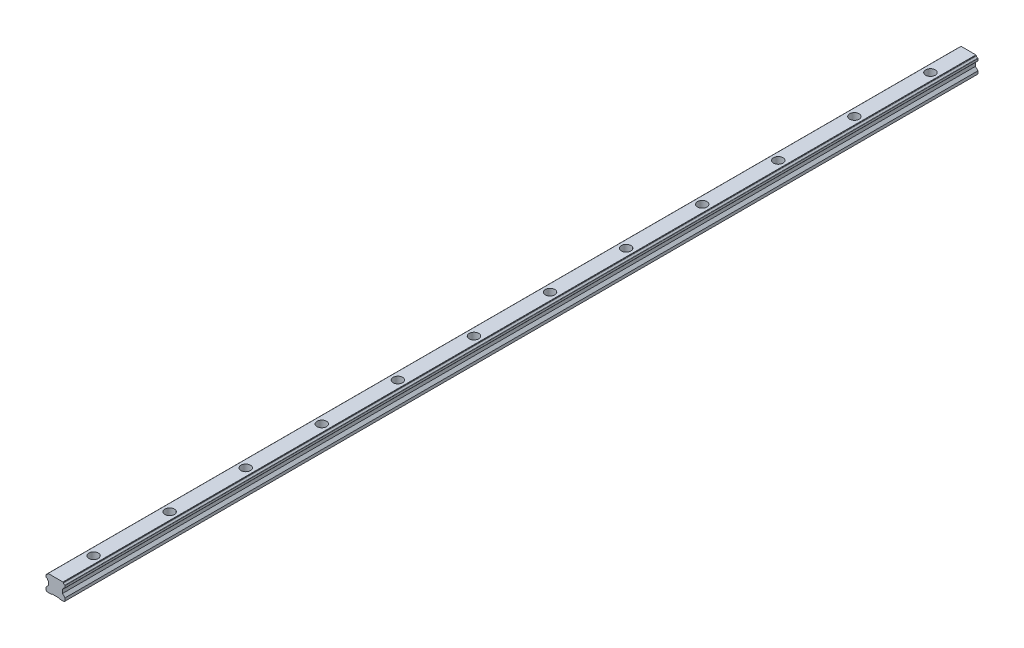
from build123d import *

# Parameters (mm, degrees)
BOSS_EXTRUDE1_DEPTH = 720
CUT_EXTRUDE1_DEPTH  = 721.116346502
CUT_EXTRUDE2_DEPTH  = 721.116346502
CUT_EXTRUDE3_DEPTH  = 721.116346502
CUT_EXTRUDE4_DEPTH  = 200
HOLE1_D             = 4.5
HOLE1_CBORE_D       = 7.5
HOLE1_CBORE_DEPTH   = 6
CHAMFER1_SIZE       = 0.7
CHAMFER2_SIZE       = 0.7
FILLET1_R           = 0.3
FILLET2_R           = 0.3
FILLET3_R           = 0.3
FILLET4_R           = 0.3
FILLET5_R           = 0.3
FILLET6_R           = 0.3
FILLET7_R           = 0.3
FILLET8_R           = 0.3
LPATTERN1_COUNT     = 12
LPATTERN1_PITCH     = 60


with BuildPart() as part:
    # Sketch1 → Boss-Extrude1 (new body)
    with BuildSketch(Plane.XY):
        with BuildLine():
            Line((7.5, -10.55), (7.5, 1.029661645))
            ThreePointArc((7.5, 1.029661645), (6.653187418, 1.325902711), (6.199900247, 2.100099753))
            Line((6.199900247, 2.100099753), (5.85, 2.45))
            Line((5.85, 2.45), (-5.85, 2.45))
            Line((-5.85, 2.45), (-6.199900248, 2.100099753))
            ThreePointArc((-6.199900248, 2.100099753), (-6.653187418, 1.325902711), (-7.5, 1.029661645))
            Line((-7.5, 1.029661645), (-7.5, -10.55))
            Line((-7.5, -10.55), (7.5, -10.55))
        make_face()
    extrude(amount=-BOSS_EXTRUDE1_DEPTH)

    # Sketch2 → Cut-Extrude1 (cut, through all)
    with BuildSketch(Plane(origin=(0, 0, -720), x_dir=(-1, 0, 0), z_dir=(0, 0, -1))):
        with BuildLine():
            Line((-7.5, -1.029661645), (-7.5, -7.6))
            Line((-7.5, -7.6), (-5.5, -5.6))
            Line((-5.5, -5.6), (-5.5, -2.8))
            Line((-5.5, -2.8), (-6.199900248, -2.100099752))
            ThreePointArc((-6.199900248, -2.100099752), (-6.653187419, -1.325902711), (-7.5, -1.029661645))
        make_face()
    extrude(amount=-CUT_EXTRUDE1_DEPTH, mode=Mode.SUBTRACT)

    # Sketch3 → Cut-Extrude2 (cut, through all)
    with BuildSketch(Plane(origin=(0, 0, -720), x_dir=(-1, 0, 0), z_dir=(0, 0, -1))):
        with BuildLine():
            Line((6.199900248, -2.100099752), (5.5, -2.8))
            Line((5.5, -2.8), (5.5, -5.6))
            Line((5.5, -5.6), (7.5, -7.6))
            Line((7.5, -7.6), (7.5, -1.029661645))
            ThreePointArc((7.5, -1.029661645), (6.653187419, -1.325902711), (6.199900248, -2.100099752))
        make_face()
    extrude(amount=-CUT_EXTRUDE2_DEPTH, mode=Mode.SUBTRACT)

    # Sketch4 → Cut-Extrude3 (cut, through all)
    with BuildSketch(Plane(origin=(0, 0, -720), x_dir=(-1, 0, 0), z_dir=(0, 0, -1))):
        Polygon((-3.35, -10.55), (3.35, -10.55), (2.85, -10.05), (-2.85, -10.05), align=None)
    extrude(amount=-CUT_EXTRUDE3_DEPTH, mode=Mode.SUBTRACT)

    # Sketch5 → Cut-Extrude4 (cut)
    with BuildSketch(Plane(origin=(0, 0, -720), x_dir=(-1, 0, 0), z_dir=(0, 0, -1))):
        with BuildLine():
            Line((-5.75, -10.55), (-4.95, -10.55))
            ThreePointArc((-4.95, -10.55), (-5.35, -10.35), (-5.75, -10.55))
        make_face()
    extrude(amount=-CUT_EXTRUDE4_DEPTH, mode=Mode.SUBTRACT)

    # Hole1 (through all)
    with Locations(Plane(origin=(0, 2.45, 0), x_dir=(-1, 0, 0), z_dir=(0, 1, 0))):
        with Locations((0, -30)):
            hole1 = CounterBoreHole(HOLE1_D / 2, HOLE1_CBORE_D / 2, HOLE1_CBORE_DEPTH)

    # Chamfer1
    chamfer1_edges = [part.edges().sort_by_distance(p)[0] for p in [
        (-7.5, -10.55, -360),
    ]]
    chamfer(chamfer1_edges, length=CHAMFER1_SIZE)

    # Chamfer2
    chamfer2_edges = [part.edges().sort_by_distance(p)[0] for p in [
        (7.5, -10.55, -360),
    ]]
    chamfer(chamfer2_edges, length=CHAMFER2_SIZE)

    # Fillet1
    fillet1_edges = [part.edges().sort_by_distance(p)[0] for p in [
        (7.5, 1.029661645, -360),
    ]]
    fillet(fillet1_edges, radius=FILLET1_R)

    # Fillet2
    fillet2_edges = [part.edges().sort_by_distance(p)[0] for p in [
        (-7.5, 1.029661645, -360),
    ]]
    fillet(fillet2_edges, radius=FILLET2_R)

    # Fillet3
    fillet3_edges = [part.edges().sort_by_distance(p)[0] for p in [
        (7.5, -1.029661645, -360),
    ]]
    fillet(fillet3_edges, radius=FILLET3_R)

    # Fillet4
    fillet4_edges = [part.edges().sort_by_distance(p)[0] for p in [
        (6.199900247, 2.100099753, -360),
    ]]
    fillet(fillet4_edges, radius=FILLET4_R)

    # Fillet5
    fillet5_edges = [part.edges().sort_by_distance(p)[0] for p in [
        (-7.5, -1.029661645, -360),
    ]]
    fillet(fillet5_edges, radius=FILLET5_R)

    # Fillet6
    fillet6_edges = [part.edges().sort_by_distance(p)[0] for p in [
        (-6.199900248, -2.100099752, -360),
    ]]
    fillet(fillet6_edges, radius=FILLET6_R)

    # Fillet7
    fillet7_edges = [part.edges().sort_by_distance(p)[0] for p in [
        (6.199900248, -2.100099752, -360),
    ]]
    fillet(fillet7_edges, radius=FILLET7_R)

    # Fillet8
    fillet8_edges = [part.edges().sort_by_distance(p)[0] for p in [
        (-6.199900248, 2.100099753, -360),
    ]]
    fillet(fillet8_edges, radius=FILLET8_R)

    # LPattern1: Hole1 ×12
    with Locations(*[(0, 0, -i * LPATTERN1_PITCH) for i in range(1, LPATTERN1_COUNT)]):
        add(hole1, mode=Mode.SUBTRACT)


solid = part.part
